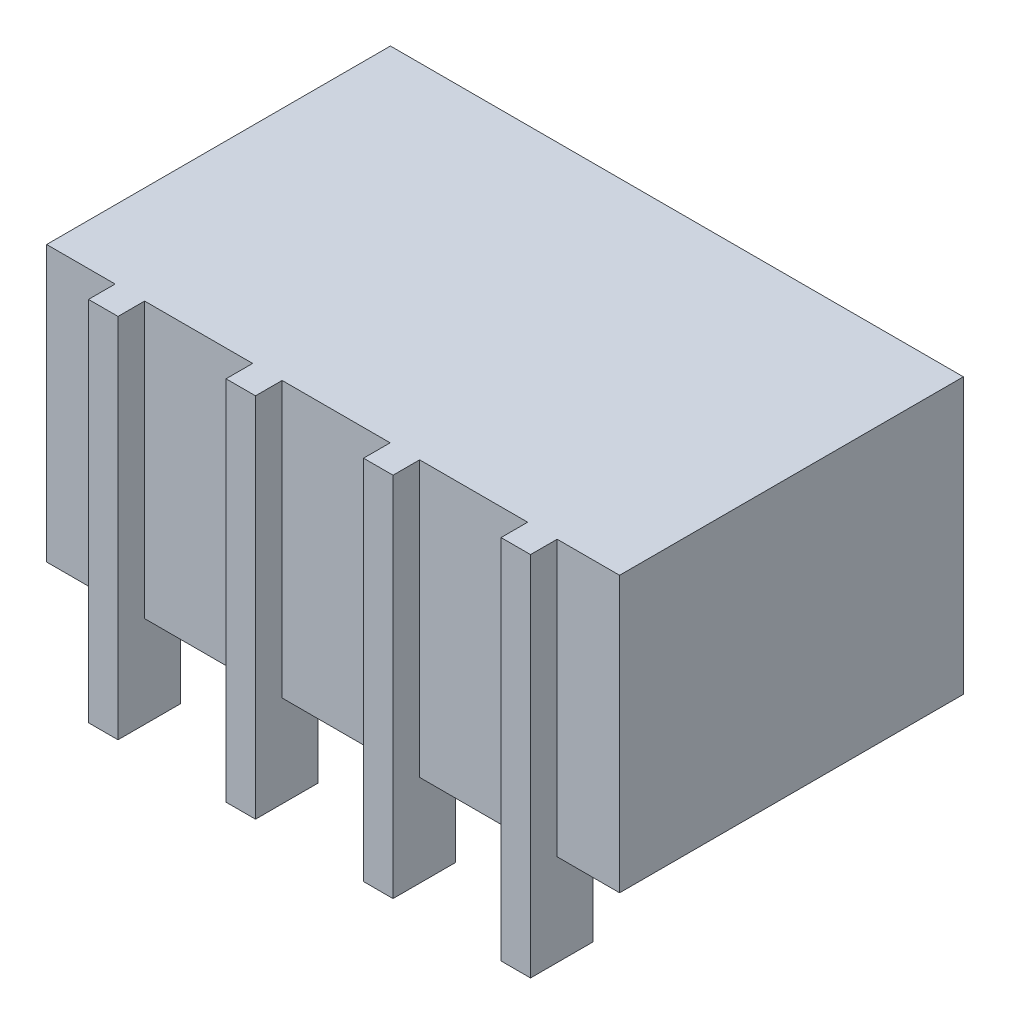
from build123d import *

# Parameters (mm, degrees)
SKETCH_1_W          = 12.5
SKETCH_1_H          = 6
EXTRUDE_1_DEPTH     = 7.5
SKETCH_2_W          = 11.342894438
SKETCH_2_H          = 4.477163802
SKETCH_2_R          = 0.480353021
SKETCH_2_R_2        = 0.517183851
SKETCH_2_R_3        = 0.582724364
SKETCH_2_R_4        = 0.500500501
CUT_EXTRUDE_1_DEPTH = 5
SKETCH_3_W          = 0.643352529
SKETCH_3_H          = 1.364086891
EXTRUDE_2_DEPTH     = 8


with BuildPart() as part:
    # 草图1 → 拉伸1 (new body)
    with BuildSketch(Plane.XY):
        with Locations((5.032975889, 1.613598403)):
            Rectangle(SKETCH_1_W, SKETCH_1_H)
    extrude(amount=EXTRUDE_1_DEPTH)

    # 草图2 → 切除-拉伸1 (cut)
    with BuildSketch(Plane(origin=(0, 0, 0), x_dir=(-1, 0, 0), z_dir=(0, 0, -1))):
        with Locations((-5.104708636, 1.729550555)):
            Rectangle(SKETCH_2_W, SKETCH_2_H)
        with Locations((-7.986319653, 2.191858525)):
            Circle(SKETCH_2_R, mode=Mode.SUBTRACT)
        with Locations((-6.334668001, 2.191858525)):
            Circle(SKETCH_2_R_2, mode=Mode.SUBTRACT)
        with Locations((-4.299299299, 2.191858525)):
            Circle(SKETCH_2_R_3, mode=Mode.SUBTRACT)
        with Locations((-2.230563897, 2.191858525)):
            Circle(SKETCH_2_R_4, mode=Mode.SUBTRACT)
    extrude(amount=-CUT_EXTRUDE_1_DEPTH, mode=Mode.SUBTRACT)

    # 草图3 → 拉伸2 (add)
    with BuildSketch(Plane(origin=(0, 4.613598403, 4.886401597), x_dir=(1, 0, 0), z_dir=(0, -1, 0))):
        with Locations((6.598992375, 2.512158379)):
            Rectangle(SKETCH_3_W, SKETCH_3_H)
        with Locations((9.598992375, 2.512158379)):
            Rectangle(SKETCH_3_W, SKETCH_3_H)
        with Locations((3.598992375, 2.512158379)):
            Rectangle(SKETCH_3_W, SKETCH_3_H)
        with Locations((0.598992376, 2.512158379)):
            Rectangle(SKETCH_3_W, SKETCH_3_H)
    extrude(amount=EXTRUDE_2_DEPTH)


solid = part.part
